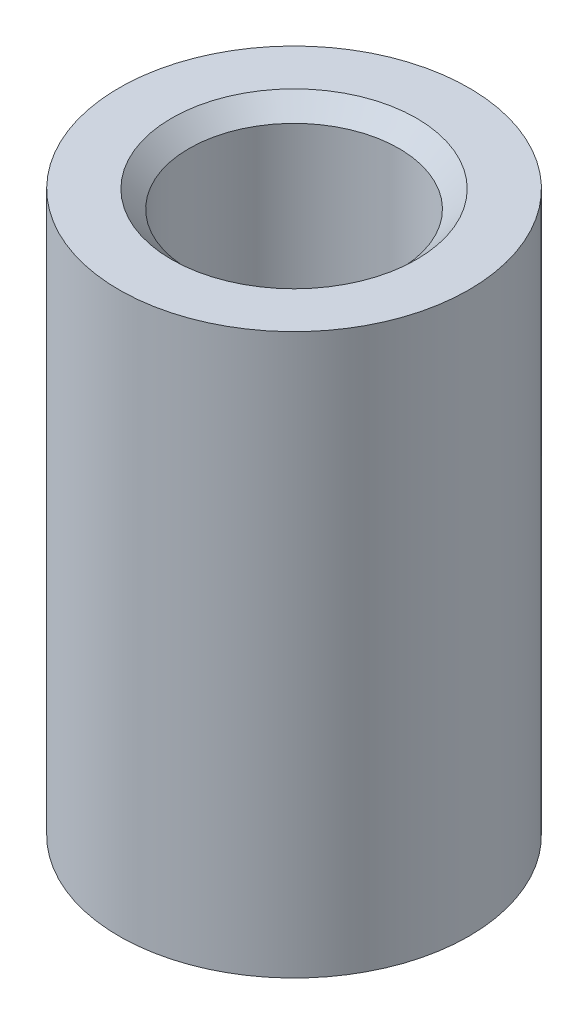
from build123d import *

# Parameters (mm, degrees)
SKETCH1_W          = 5
SKETCH1_H          = 16
SKETCH2_R          = 3
CUT_EXTRUDE1_DEPTH = 10
CHAMFER1_SIZE      = 0.5


with BuildPart() as part:
    # Sketch1 → Revolve1 (revolve)
    with BuildSketch(Plane.XY):
        with Locations((2.5, -8)):
            Rectangle(SKETCH1_W, SKETCH1_H)
    revolve(axis=Axis((0, -264.304461942, 0), (0, 1, 0)))

    # Sketch2 → Cut-Extrude1 (cut)
    with BuildSketch(Plane(origin=(0, 0, 0), x_dir=(1, 0, 0), z_dir=(0, 1, 0))):
        with Locations(Location((0, 0, 0), (0, 0, 180))):
            Circle(SKETCH2_R)
    extrude(amount=-CUT_EXTRUDE1_DEPTH, mode=Mode.SUBTRACT)

    # Chamfer1
    chamfer1_edges = [part.edges().sort_by_distance(p)[0] for p in [
        (3, 0, 0),
    ]]
    chamfer(chamfer1_edges, length=CHAMFER1_SIZE)


solid = part.part
